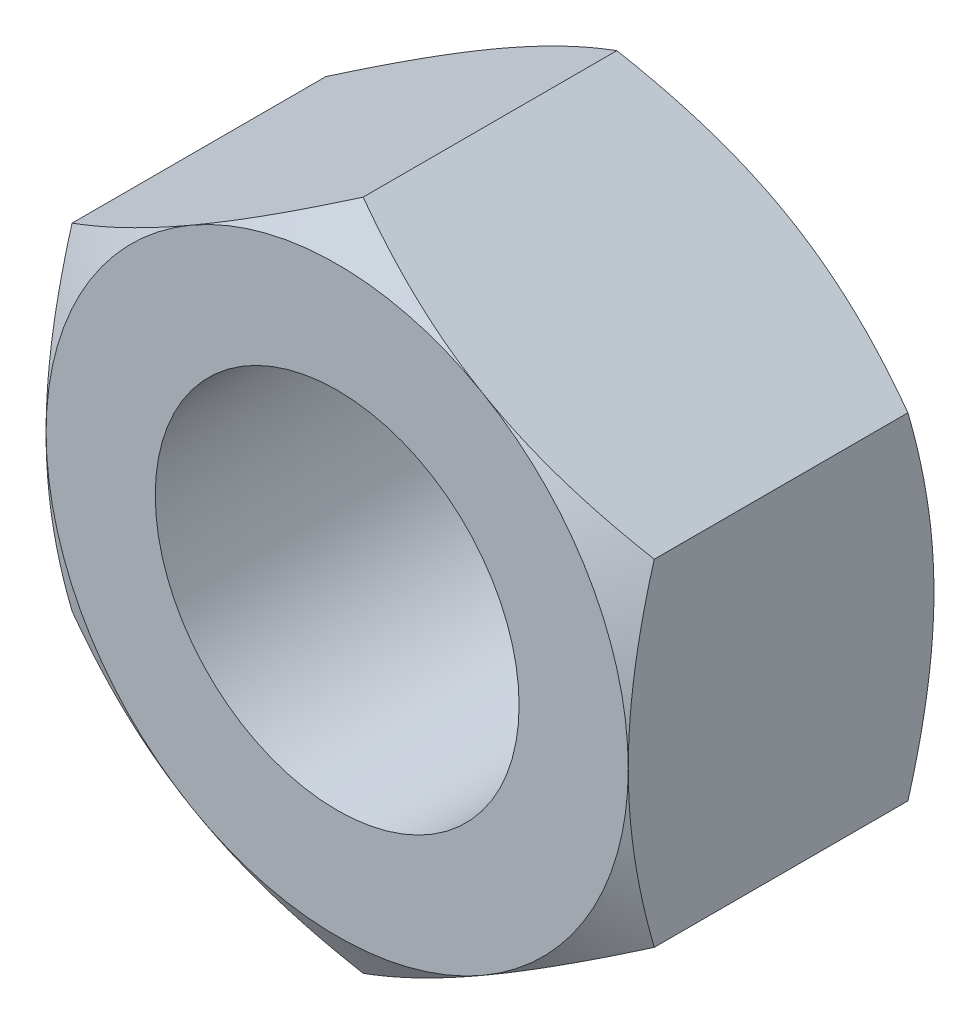
from build123d import *

# Parameters (mm, degrees)
EXTRUDE_1_DEPTH     = 8.4
SKETCH_5_R          = 5
CUT_EXTRUDE_1_DEPTH = 15.828800806
SKETCH_6_OUTSIDE_W  = 369.578
SKETCH_6_OUTSIDE_H  = 372.054
SKETCH_6_OUTSIDE_R  = 8
CUT_EXTRUDE_2_DEPTH = 100
CUT_EXTRUDE_2_DRAFT = -60
SKETCH_7_OUTSIDE_W  = 369.578
SKETCH_7_OUTSIDE_H  = 372.054
SKETCH_7_OUTSIDE_R  = 8
CUT_EXTRUDE_3_DEPTH = 100
CUT_EXTRUDE_3_DRAFT = -60


with BuildPart() as part:
    # 草图1 → 凸台-拉伸1 (new body)
    with BuildSketch(Plane.XY):
        Polygon((0, 9.237604307), (-8, 4.618802154), (-8, -4.618802154), (0, -9.237604307), (8, -4.618802154), (8, 4.618802154), align=None)
    extrude(amount=EXTRUDE_1_DEPTH)

    # 草图5 → 切除-拉伸1 (cut, through all)
    with BuildSketch(Plane.XY.offset(8.4)):
        Circle(SKETCH_5_R)
    extrude(amount=-CUT_EXTRUDE_1_DEPTH, mode=Mode.SUBTRACT)


with BuildPart() as cut_extrude_2_tool:
    # 草图6 outside → 切除-拉伸2 (with draft: the straight prism first)
    with BuildSketch(Plane.XY.offset(8.4)):
        Rectangle(SKETCH_6_OUTSIDE_W, SKETCH_6_OUTSIDE_H)
        Circle(SKETCH_6_OUTSIDE_R, mode=Mode.SUBTRACT)
    extrude(amount=-CUT_EXTRUDE_2_DEPTH)
    # 切除-拉伸2: the draft: its side faces are tilted about the plane it starts from
    cut_extrude_2_sides = [cut_extrude_2_tool.faces().sort_by_distance(p)[0] for p in [
        (0, -186.027, -41.6),
        (184.789, 0, -41.6),
        (0, 186.027, -41.6),
        (-184.789, 0, -41.6),
        (-8, 0, -41.6),
    ]]
    draft(cut_extrude_2_sides, Plane.XY.offset(8.4), CUT_EXTRUDE_2_DRAFT)


with BuildPart() as part_1:
    add(part.part)

    # 切除-拉伸2: cut by cut_extrude_2_tool
    add(cut_extrude_2_tool.part, mode=Mode.SUBTRACT)


with BuildPart() as cut_extrude_3_tool:
    # 草图7 outside → 切除-拉伸3 (with draft: the straight prism first)
    with BuildSketch(Plane(origin=(0, 0, 0), x_dir=(-1, 0, 0), z_dir=(0, 0, -1))):
        Rectangle(SKETCH_7_OUTSIDE_W, SKETCH_7_OUTSIDE_H)
        Circle(SKETCH_7_OUTSIDE_R, mode=Mode.SUBTRACT)
    extrude(amount=-CUT_EXTRUDE_3_DEPTH)
    # 切除-拉伸3: the draft: its side faces are tilted about the plane it starts from
    cut_extrude_3_sides = [cut_extrude_3_tool.faces().sort_by_distance(p)[0] for p in [
        (0, -186.027, 50),
        (-184.789, 0, 50),
        (0, 186.027, 50),
        (184.789, 0, 50),
        (8, 0, 50),
    ]]
    draft(cut_extrude_3_sides, Plane(origin=(0, 0, 0), x_dir=(-1, 0, 0), z_dir=(0, 0, -1)), CUT_EXTRUDE_3_DRAFT)


with BuildPart() as part_2:
    add(part_1.part)

    # 切除-拉伸3: cut by cut_extrude_3_tool
    add(cut_extrude_3_tool.part, mode=Mode.SUBTRACT)


solid = part_2.part
